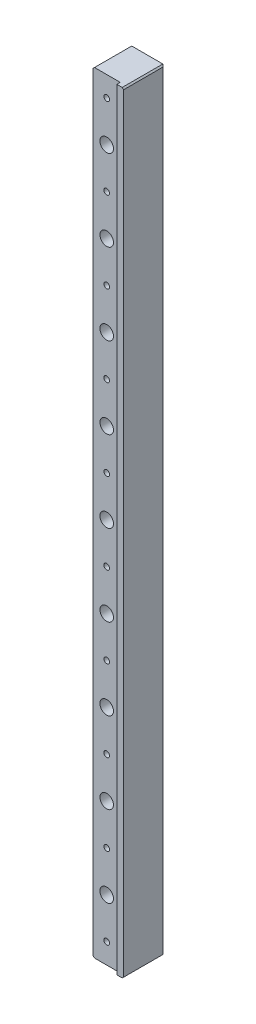
from build123d import *

# Parameters (mm, degrees)
SKETCH1_W                                           = 25
SKETCH1_H                                           = 570
EXTRUDE1_DEPTH                                      = 15
CHAMFER1_SIZE                                       = 1
SKETCH_1_W                                          = 20
SKETCH_1_H                                          = 570
CUT_EXTRUDE1_DEPTH                                  = 2.5
CHAMFER2_SIZE                                       = 1
M5_TAPPED_HOLE1_D                                   = 4.2
M5_TAPPED_HOLE1_DEPTH                               = 14
M5_TAPPED_HOLE1_TIP                                 = 1.2618073
HOLE_SIZE_PER_SOCKET_HEAD_CAP_SCREW_TYP_D           = 5.5
HOLE_SIZE_PER_SOCKET_HEAD_CAP_SCREW_TYP_CBORE_D     = 10
HOLE_SIZE_PER_SOCKET_HEAD_CAP_SCREW_TYP_CBORE_DEPTH = 8
LPATTERN1_COUNT                                     = 9
LPATTERN1_PITCH                                     = 60


with BuildPart() as part:
    # Sketch1 → Extrude1 (new, symmetric)
    with BuildSketch(Plane.XY):
        Rectangle(SKETCH1_W, SKETCH1_H)
    extrude(amount=EXTRUDE1_DEPTH, both=True)

    # Chamfer1
    chamfer1_edges = [part.edges().sort_by_distance(p)[0] for p in [
        (-12.5, 285, 0),
        (12.5, 285, 0),
        (12.5, -285, 0),
        (-12.5, -285, 0),
    ]]
    chamfer(chamfer1_edges, length=CHAMFER1_SIZE)

    # 草图1 → Cut-Extrude1 (cut)
    with BuildSketch(Plane.XY.offset(15)):
        with Locations((-2.5, 0)):
            Rectangle(SKETCH_1_W, SKETCH_1_H)
    extrude(amount=-CUT_EXTRUDE1_DEPTH, mode=Mode.SUBTRACT)

    # Chamfer2
    chamfer2_edges = [part.edges().sort_by_distance(p)[0] for p in [
        (12.5, 0, -15),
        (-12.5, 0, -15),
    ]]
    chamfer(chamfer2_edges, length=CHAMFER2_SIZE)

    # M5 Tapped Hole1
    with Locations(Plane.XY.offset(12.5)):
        with Locations((-2.5, -270), (-2.5, -210), (-2.5, -150), (-2.5, -90), (-2.5, -30), (-2.5, 30), (-2.5, 90), (-2.5, 150), (-2.5, 210), (-2.5, 270)):
            Hole(M5_TAPPED_HOLE1_D / 2, depth=M5_TAPPED_HOLE1_DEPTH)
            with Locations((0, 0, -(M5_TAPPED_HOLE1_DEPTH + M5_TAPPED_HOLE1_TIP / 2))):  # 118° drill point
                Cone(0, M5_TAPPED_HOLE1_D / 2, M5_TAPPED_HOLE1_TIP, mode=Mode.SUBTRACT)

    # Hole size (per socket head cap screw type)1 (through all)
    with Locations(Plane.XY.offset(12.5)):
        with Locations((-2.5, 240)):
            hole_size_per_socket_head_cap_screw_typ = CounterBoreHole(HOLE_SIZE_PER_SOCKET_HEAD_CAP_SCREW_TYP_D / 2, HOLE_SIZE_PER_SOCKET_HEAD_CAP_SCREW_TYP_CBORE_D / 2, HOLE_SIZE_PER_SOCKET_HEAD_CAP_SCREW_TYP_CBORE_DEPTH)

    # LPattern1: Hole size (per socket head cap screw type)1 ×9
    with Locations(*[(0, -i * LPATTERN1_PITCH, 0) for i in range(1, LPATTERN1_COUNT)]):
        add(hole_size_per_socket_head_cap_screw_typ, mode=Mode.SUBTRACT)


solid = part.part
